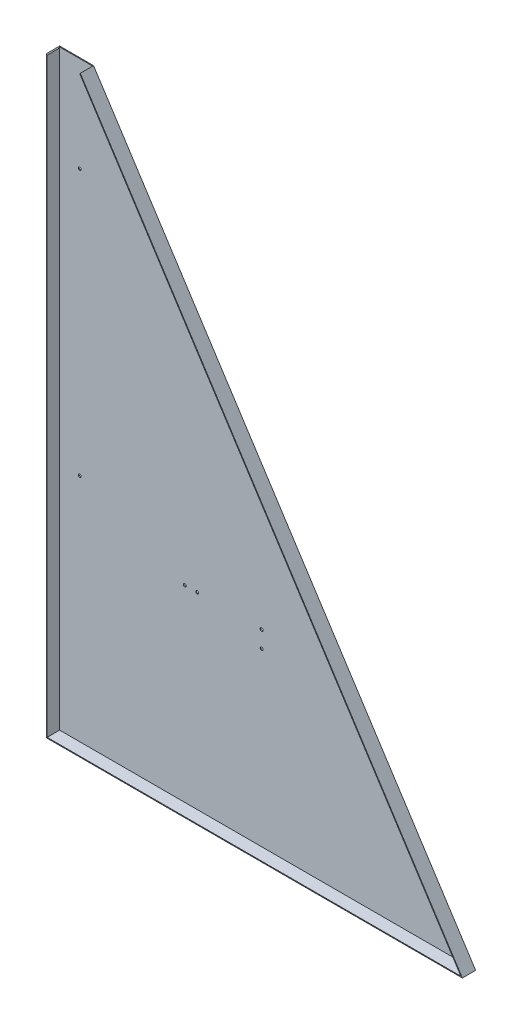
from build123d import *

# Parameters (mm, degrees)
SKETCH1_W           = 1002
SKETCH1_H           = 1427
BOSS_EXTRUDE1_DEPTH = 2
CUT_EXTRUDE1_DEPTH  = 2
SKETCH5_R           = 3.5
CUT_EXTRUDE2_DEPTH  = 40
BOSS_EXTRUDE2_DEPTH = 30
SKETCH7_R           = 3.5
CUT_EXTRUDE3_DEPTH  = 10


with BuildPart() as part:
    # Sketch1 → Boss-Extrude1 (new body)
    with BuildSketch(Plane.XY):
        Rectangle(SKETCH1_W, SKETCH1_H)
    extrude(amount=BOSS_EXTRUDE1_DEPTH)

    # Sketch2 → Cut-Extrude1 (cut)
    with BuildSketch(Plane.XY.offset(2)):
        Polygon((-419.25, 713.5), (501, -713.5), (501, 713.5), align=None)
    extrude(amount=-CUT_EXTRUDE1_DEPTH, mode=Mode.SUBTRACT)

    # Sketch5 → Cut-Extrude2 (cut)
    with BuildSketch(Plane.XY.offset(2)):
        with Locations((-197.5, -258.5)):
            Circle(SKETCH5_R)
        with Locations((-167.5, -258.5)):
            Circle(SKETCH5_R)
        with Locations((-12.5, -258.5)):
            Circle(SKETCH5_R)
        with Locations((-12.5, -298.5)):
            Circle(SKETCH5_R)
    extrude(amount=-CUT_EXTRUDE2_DEPTH, mode=Mode.SUBTRACT)

    # Sketch6 → Boss-Extrude2 (add)
    with BuildSketch(Plane.XY.offset(2)):
        Polygon((-499, 711.5), (-499, -711.5), (497.33041962, -711.5), (-420.340042889, 711.5), (-419.25, 713.5), (501, -713.5), (-501, -713.5), (-501, 713.5), align=None)
    extrude(amount=BOSS_EXTRUDE2_DEPTH)

    # Sketch7 → Cut-Extrude3 (cut)
    with BuildSketch(Plane.XY.offset(2)):
        with Locations((-450.5, 483.5)):
            Circle(SKETCH7_R)
        with Locations((-450.5, -156.5)):
            Circle(SKETCH7_R)
    extrude(amount=-CUT_EXTRUDE3_DEPTH, mode=Mode.SUBTRACT)


solid = part.part
